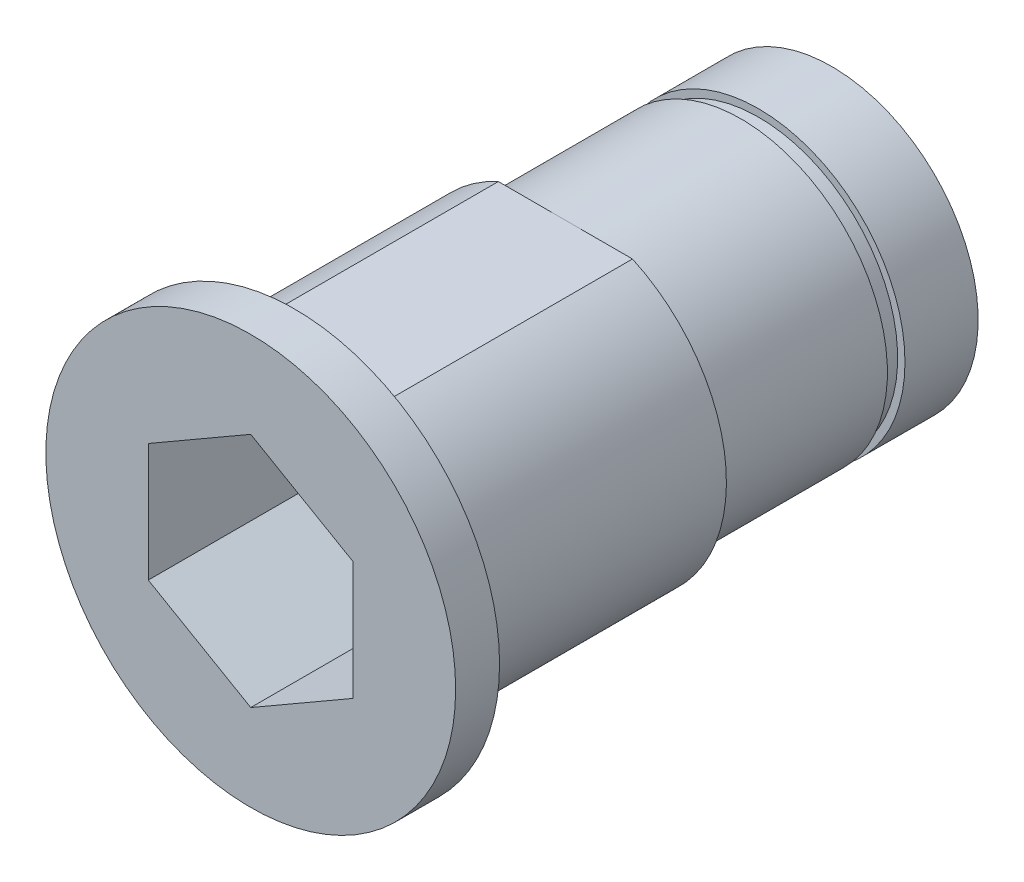
from build123d import *

# Parameters (mm, degrees)
SKETCH_1_R          = 11
SKETCH_1_R_2        = 6
EXTRUDE_1_DEPTH     = 34
SKETCH_2_R          = 14
SKETCH_2_R_2        = 7
EXTRUDE_2_DEPTH     = 3
SKETCH_3_R          = 12.01734277
SKETCH_3_R_2        = 10
CUT_EXTRUDE_1_DEPTH = 15.5
SKETCH_4_W          = 13.23621111
SKETCH_4_H          = 1.977552999
CUT_EXTRUDE_2_DEPTH = 32
CUT_EXTRUDE_3_DEPTH = 42.964270517
SKETCH_6_W          = 1
SKETCH_6_H          = 1.2
EXTRUDE_START       = 2.7
SKETCH_7_R          = 10
EXTRUDE_3_DEPTH     = 2.7


with BuildPart() as part:
    # 草图1 → 凸台-拉伸1 (new body)
    with BuildSketch(Plane.XY):
        Circle(SKETCH_1_R)
        Circle(SKETCH_1_R_2, mode=Mode.SUBTRACT)
    extrude(amount=EXTRUDE_1_DEPTH)

    # 草图2 → 凸台-拉伸2 (add)
    with BuildSketch(Plane.XY.offset(34)):
        Circle(SKETCH_2_R)
        Circle(SKETCH_2_R_2, mode=Mode.SUBTRACT)
    extrude(amount=EXTRUDE_2_DEPTH)

    # 草图3 → 切除-拉伸1 (cut)
    with BuildSketch(Plane(origin=(0, 0, 0), x_dir=(-1, 0, 0), z_dir=(0, 0, -1))):
        Circle(SKETCH_3_R)
        Circle(SKETCH_3_R_2, mode=Mode.SUBTRACT)
    extrude(amount=-CUT_EXTRUDE_1_DEPTH, mode=Mode.SUBTRACT)

    # 草图4 → 切除-拉伸2 (cut)
    with BuildSketch(Plane(origin=(0, 0, 0), x_dir=(-1, 0, 0), z_dir=(0, 0, -1))):
        with Locations((1.1977553, 10.9887765)):
            Rectangle(SKETCH_4_W, SKETCH_4_H)
    extrude(amount=-CUT_EXTRUDE_2_DEPTH, mode=Mode.SUBTRACT)

    # 草图5 → 切除-拉伸3 (cut, through all)
    with BuildSketch(Plane.XY.offset(37)):
        Polygon((7, -4.041451884), (7, 4.041451884), (0, 8.082903769), (-7, 4.041451884), (-7, -4.041451884), (0, -8.082903769), align=None)
    extrude(amount=-CUT_EXTRUDE_3_DEPTH, mode=Mode.SUBTRACT)

    # 草图6 → 切除-旋转1 (revolve, cut)
    with BuildSketch(Plane(origin=(0, 0, 0), x_dir=(1, 0, 0), z_dir=(0, 1, 0)), mode=Mode.PRIVATE) as cut_revolve_1_sk:
        with Locations((10, -2.9)):
            Rectangle(SKETCH_6_W, SKETCH_6_H)
    revolve(cut_revolve_1_sk.sketch.rotate(Axis((0, 0, -1.695132032), (0, 0, 1)), 180), axis=Axis((0, 0, -1.695132032), (0, 0, 1)), mode=Mode.SUBTRACT)

    # 草图7 → 凸台-拉伸3 (add)
    with BuildSketch(Plane(origin=(0, 0, 0), x_dir=(-1, 0, 0), z_dir=(0, 0, -1)).offset(EXTRUDE_START)):
        Circle(SKETCH_7_R)
        Polygon((7, -4.041451884), (7, 4.041451884), (0, 8.082903769), (-7, 4.041451884), (-7, -4.041451884), (0, -8.082903769), align=None, mode=Mode.SUBTRACT)
    extrude(amount=-EXTRUDE_3_DEPTH)


solid = part.part
